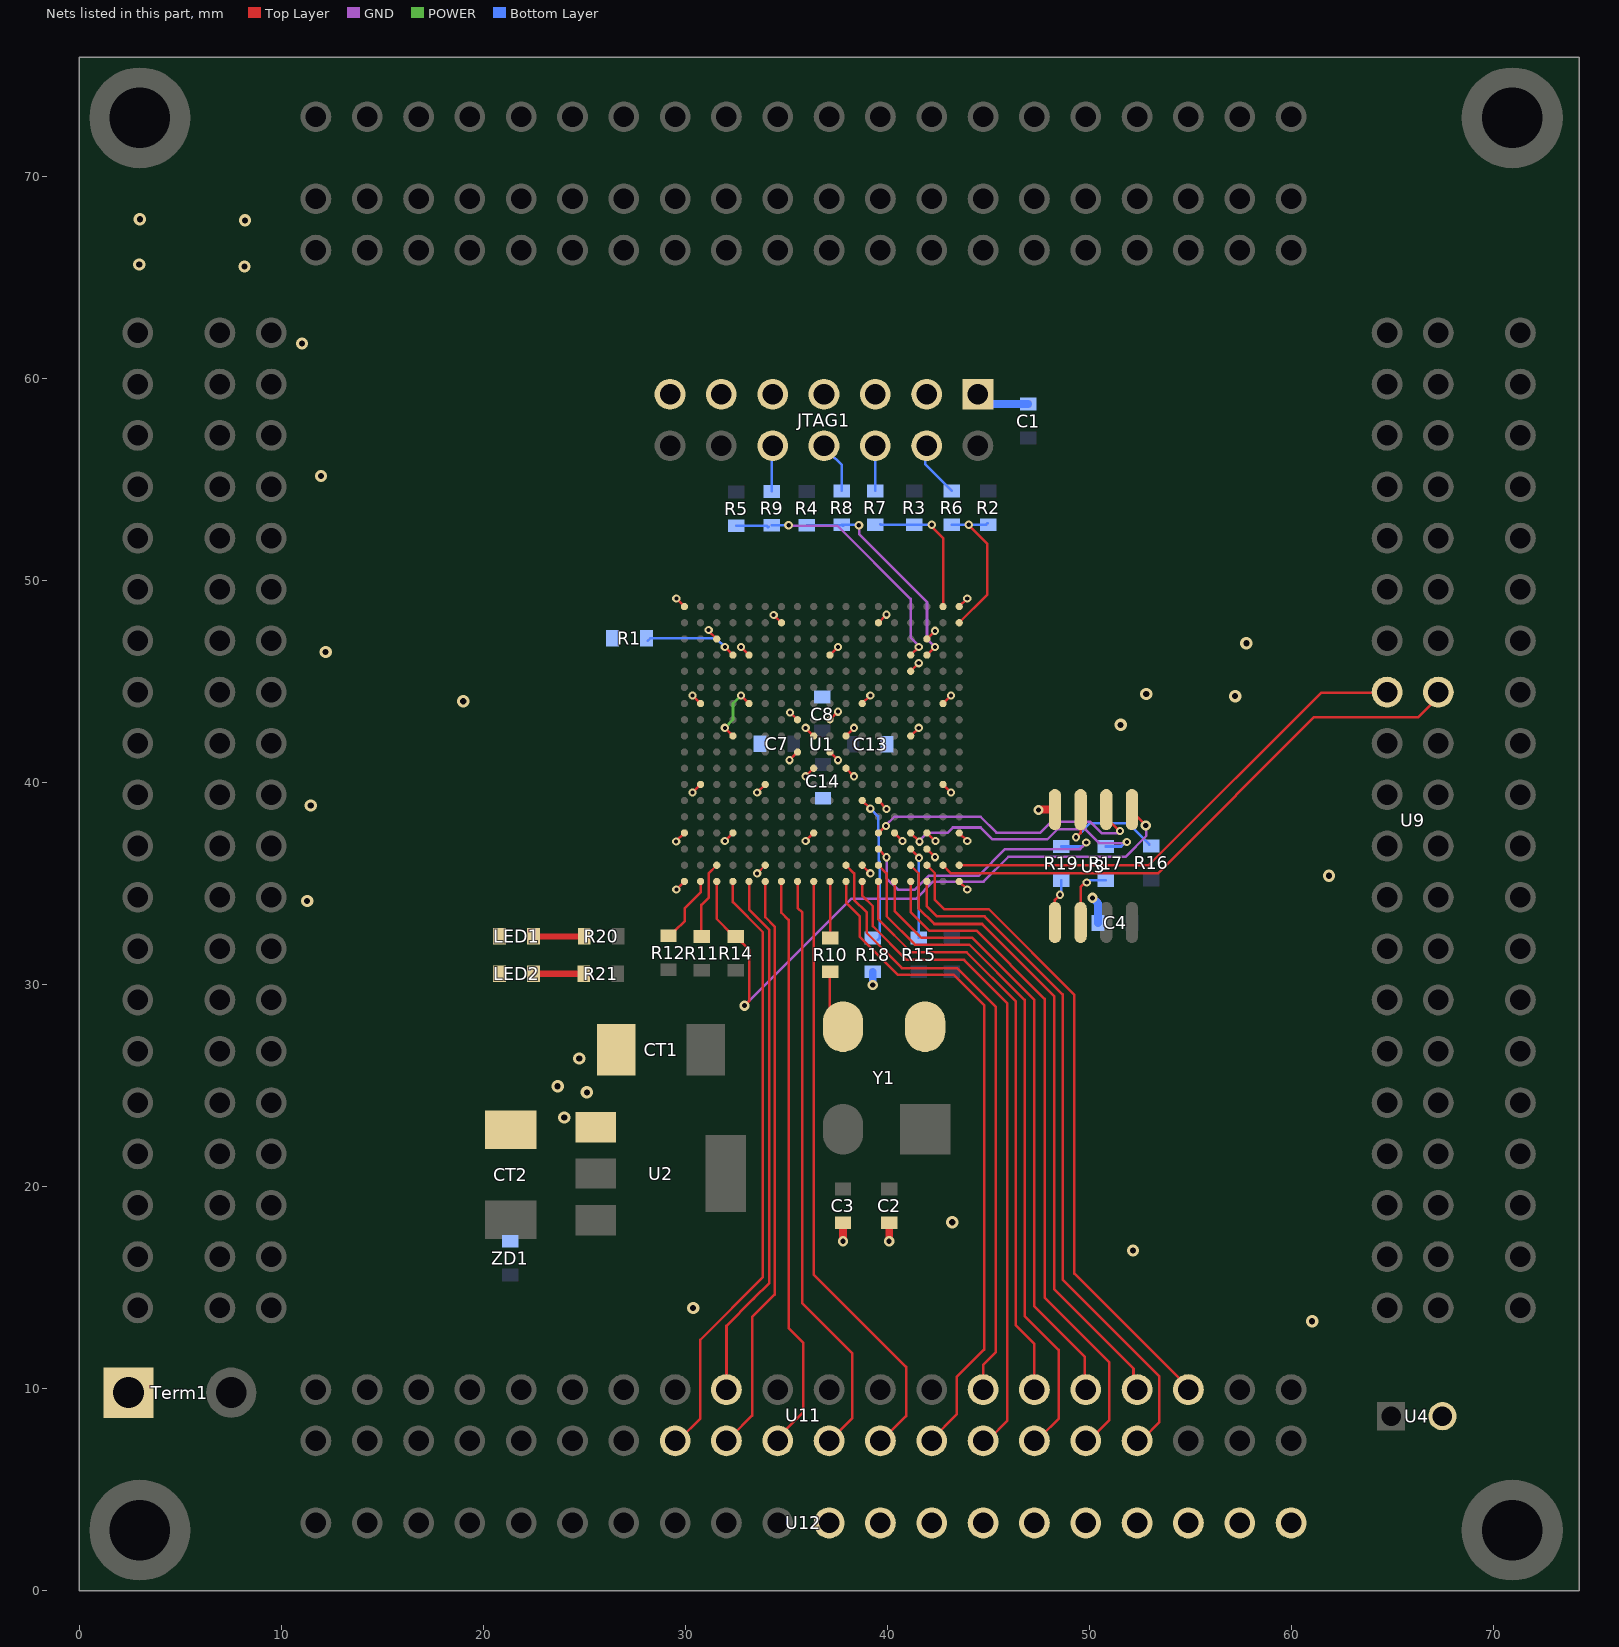
[diagram p0: the nets of this part, all layers, seen from the top]
# Altium PCB MISC103828.PcbDoc (part 4 of 4)
Units mm, origin at the board's own origin, x right, y up, seen from the top; angles counter-clockwise.
Board outline 74.24 x 75.89 mm, 4 copper layers (Top Layer, GND, POWER, Bottom Layer); 49 components, 246 nets, 670 pads, 283 vias.

## Via types
v1: diameter 0.406, hole 0.203, Top Layer to Bottom Layer, 221 vias
v2: diameter 0.61, hole 0.305, Top Layer to Bottom Layer, 43 vias
v3: diameter 0.508, hole 0.254, Top Layer to Bottom Layer, 16 vias
v4: diameter 0.432, hole 0.229, Top Layer to Bottom Layer, 3 vias

## Nets (pads, with @x,y where several pads share a name; then routed paths per layer and width w, separated by ;. In a path a pad name is that pad's centre, name@x,y a point inside that pad or via, vN(x,y) a via of type N, cw(c..) or ccw(c..) an arc to the next point about the centre after c; other vN are vias at no path point) (continued)
F_U11: U1.U11 U11.28 | length 30.9
  Top Layer w0.127: U1.U11@37.947,35.903 38.351,35.499 38.351,34.191 38.964,33.579 38.964,32.563 40.716,30.81 43.434,30.81 45.364,28.88 45.364,11.811 44.729,11.176 U11.28@44.729,9.957
F_U13: U1.U13 U11.29 | length 34
  Top Layer w0.127: U1.U13@39.547,35.903 39.951,35.499 39.951,33.378 41.351,31.979 44.044,31.979 46.787,29.235 46.787,15.037 ; 46.787,14.961 46.787,15.037 ; U11.29@47.6,7.645 48.463,8.509 48.463,11.913 46.787,13.589 46.787,15.037
F_U15: U1.U15 U11.34 | length 31.8
  Top Layer w0.127: U1.U15@41.147,35.903 41.543,35.508 41.543,33.768 42.316,32.995 44.679,32.995 48.26,29.413 48.26,14.91 52.172,10.998 U11.34@52.172,10.033
F_U16: U1.U16 U11.36 | length 32.2
  Top Layer w0.127: U1.U16@41.947,35.903 42.343,35.508 42.343,34.187 42.799,33.731 45.009,33.731 49.251,29.489 49.251,15.697 U11.36@54.686,10.262
F_U17: U1.U17 U9.16 | length 28.3
  Top Layer w0.127: U1.U17@42.747,35.903 43.151,35.499 53.381,35.499 61.112,43.231 66.269,43.231 U9.16@67.285,44.247
F_U18: U1.U18 U9.15 | length 24.7
  Top Layer w0.127: U1.U18@43.547,35.903 52.921,35.903 61.468,44.45 U9.15@64.668,44.45
F_V4: U1.V4 U11.15 | length 29.9
  Top Layer w0.127: U11.15@29.693,7.493 30.734,8.534 30.734,12.421 33.833,15.519 33.833,32.588 32.347,34.074 U1.V4@32.347,35.103
F_V5: U1.V5 U11.18 | length 26.4
  Top Layer w0.127: U11.18@32.029,9.957 32.029,13.106 33.35,14.427 33.401,14.478 34.138,15.215 34.138,32.715 33.147,33.705 U1.V5@33.147,35.103
F_V6: U1.V6 U11.17 | length 28.5
  Top Layer w0.127: U11.17@32.309,7.671 33.299,8.661 33.299,13.538 34.417,14.656 34.417,32.868 33.947,33.337 U1.V6@33.947,35.103
F_V7: U1.V7 U11.19 | length 28.1
  Top Layer w0.127: U1.V7@34.747,35.103 34.747,33.553 35.103,33.198 35.103,13.005 35.839,12.268 35.839,8.839 U11.19@34.849,7.849
F_V8: U1.V8 U11.21 | length 28.9
  Top Layer w0.127: U1.V8@35.547,35.103 35.547,33.795 35.789,33.553 35.789,14.757 ; 35.789,14.63 35.789,14.757 ; U11.21@37.516,7.798 38.252,8.534 38.252,11.76 35.789,14.224 35.789,14.757
F_V9: U1.V9 U11.23 | length 29.7
  Top Layer w0.127: 36.347,16.459 36.347,16.51 ; U1.V9@36.347,35.103 36.347,16.51 ; U11.23@39.98,7.696 40.919,8.636 40.919,11.074 36.347,15.646 36.347,16.51
F_V11: U1.V11 U11.25 | length 33.2
  Top Layer w0.127: U1.V11@37.947,35.103 37.947,34.062 38.633,33.376 38.633,32.36 40.513,30.48 43.282,30.48 44.78,28.981 44.78,11.938 43.434,10.592 43.434,8.738 U11.25@42.164,7.468
F_V12: U1.V12 U11.27 | length 32.6
  Top Layer w0.127: U1.V12@38.747,35.103 38.747,34.405 39.268,33.884 39.268,32.893 40.945,31.217 43.79,31.217 45.923,29.083 45.923,8.407 U11.27@45.034,7.518
F_V13: U1.V13 U11.30 | length 30
  Top Layer w0.127: U1.V13@39.547,35.103 39.547,33.224 41.173,31.598 43.917,31.598 46.355,29.159 46.355,13.716 ; 46.355,13.589 46.355,13.716 ; U11.30@47.269,10.084 47.269,12.217 46.355,13.132 46.355,13.716
F_V14: U1.V14 U11.32 | length 30.3
  Top Layer w0.127: U1.V14@40.347,35.103 40.347,33.643 41.681,32.309 44.196,32.309 47.269,29.235 47.269,14.072 49.759,11.582 U11.32@49.759,10.16
F_V15: U1.V15 U11.31 | length 33.4
  Top Layer w0.127: U1.V15@41.147,35.103 41.147,33.579 42.062,32.664 44.399,32.664 47.777,29.286 47.777,14.503 50.978,11.303 50.978,8.458 U11.31@50.063,7.544
F_V16: U1.V16 U11.33 | length 34
  Top Layer w0.127: U1.V16@41.947,35.103 41.947,33.872 42.443,33.376 44.806,33.376 48.666,29.515 48.666,15.392 53.442,10.617 53.442,8.331 U11.33@52.68,7.569
FPGA_CCLK: R17.1 U1.R15 | length 13
  Top Layer w0.127: U1.R15@41.147,37.503 v1(41.58,37.071)
  GND w0.127: v1(41.58,37.071) 41.547,37.103 41.947,37.503 42.53,37.503 42.596,37.503 42.964,37.503 43.231,37.77 44.602,37.77 45.187,37.186 47.904,37.186 48.4,37.681 49.797,37.681 50.495,36.982 51.765,36.982 v1(51.841,37.059)
  Bottom Layer w0.127: R17.1@50.8,36.83 51.562,36.83 v1@51.765,37.033
FPGA_CSO_B: R14.2 U1.V3 U3.1 | length 31.8
  Top Layer w0.127: U1.V3@31.547,35.103 31.547,33.248 32.309,32.487 R14.2@32.512,32.487 ; R14.2@32.487,32.385 33.147,31.725 33.147,29.185 v3(32.918,28.956) ; U3.1@52.095,38.659 52.095,38.557 v3(52.781,37.871)
  GND w0.127: v3(32.918,28.956) 38.202,34.239 41.402,34.239 42.26,35.097 44.749,35.097 45.974,36.322 51.765,36.322 52.807,37.363 v3@52.807,37.821
FPGA_DIN: U1.R13 U3.2 | length 14.4
  Top Layer w0.127: U1.R13@39.547,37.503 39.561,37.503 v1@39.878,37.821 ; v1(39.929,37.846) v1@39.954,37.821 ; U3.2@50.825,38.659 50.825,38.252 v1@51.46,37.617
  GND w0.127: v1(39.929,37.846) v1@39.954,37.821 ; v1@39.929,37.897 40.335,38.303 44.602,38.303 45.39,37.516 ; 45.39,37.51 47.543,37.51 48.082,38.049 50.038,38.049 50.597,37.49 51.41,37.49 v1(51.511,37.592)
FPGA_INIT_B: R11.2 U1.U3 | length 3.7
  Top Layer w0.127: R11.2@30.836,32.512 30.785,32.563 30.785,33.934 31.143,34.293 31.143,35.499 U1.U3@31.547,35.903
FPGA_M0: R15.2 U1.T15 | length 4.5
  Top Layer w0.127: U1.T15@41.147,36.703 41.554,36.296 v1(41.554,36.271)
  Bottom Layer w0.127: R15.2@41.554,32.309 v1@41.554,36.22
FPGA_M1: R18.2 U1.N12 | length 7.3
  Top Layer w0.127: U1.N12@38.747,39.103 v1(39.147,38.703)
  Bottom Layer w0.127: v1(39.147,38.703) 39.535,38.316 39.535,38.049 39.535,37.338 39.56,37.313 39.56,36.134 39.611,36.083 39.611,32.296 R18.2@39.522,32.207
FPGA_MOSI: R19.1 U1.T13 | length 14
  Top Layer w0.127: U1.T13@39.547,36.703 v1(39.954,36.297)
  GND w0.127: v1(39.954,36.297) 39.954,35.255 40.513,34.696 41.351,34.696 42.037,35.382 44.501,35.382 45.822,36.703 49.53,36.703 v1@49.86,37.033 ; v1@49.797,37.033 v1(49.835,37.033)
  Bottom Layer w0.127: R19.1@48.59,36.83 49.632,36.83 v1@49.784,36.982
GND: C1.1 C2.1 C3.1 C4.2 C7.1 C8.1 C13.1 C14.1 CT1.2 CT2.2 JTAG1.1 JTAG1.3 JTAG1.5 JTAG1.7 JTAG1.9 JTAG1.11 JTAG1.13 LED1.K LED2.K R1.1 R18.1 Term1.1 U1.A1 U1.A18 U1.B7 U1.B13 U1.C3 U1.C16 U1.D5 U1.D10 U1.E15 U1.G2 U1.G5 U1.G12 U1.G17 U1.H8 U1.H10 U1.J4 U1.J9 U1.J11 U1.J15 U1.K8 U1.K10 U1.L9 U1.L11 U1.M2 U1.M6 U1.M17 U1.N13 U1.R1 U1.R4 U1.R9 U1.R14 U1.R16 U1.R18 U1.T16 U1.U6 U1.U12 U1.V1 U1.V18 U2.1 U3.4 U4.2 U12.11 U12.12 U12.13 U12.14 U12.15 U12.16 U12.17 U12.18 U12.19 U12.20 Y1.2 ZD1.1 | length 30.4
  Top Layer w0.127: v1(29.54,37.084) 29.54,37.096 U1.R1@29.947,37.503 ; v1(29.547,34.703) U1.V1@29.947,35.103 ; v1(29.547,49.103) U1.A1@29.947,48.703 ; v1(30.347,39.503) U1.M2@30.747,39.903 ; v1(30.347,44.303) U1.G2@30.747,43.903 ; v1(31.147,47.542) 31.147,47.503 U1.C3@31.547,47.103 ; v1(31.947,37.103) U1.R4@32.347,37.503 ; v1(31.947,42.703) U1.J4@32.347,42.303 ; v1(32.747,44.303) U1.G5@33.147,43.903 ; v1(32.747,46.703) U1.D5@33.147,46.303 ; v1(33.547,35.503) U1.U6@33.947,35.903 ; v1(33.547,39.503) U1.M6@33.947,39.903 ; v1(34.366,48.285) U1.B7@34.747,47.903 ; v1(35.147,41.103) U1.K8@35.547,41.503 ; v1(35.179,43.459) 35.179,43.472 U1.H8@35.547,43.103 ; v1(35.947,37.103) U1.R9@36.347,37.503 ; v1(35.947,40.303) U1.L9@36.347,40.703 ; v1(35.947,42.703) U1.J9@36.347,42.303 ; U1.K10@37.147,41.503 v1(37.547,41.103) ; U1.H10@37.147,43.103 v1(37.547,43.503) ; U1.D10@37.147,46.303 v1(37.547,46.703) ; U1.L11@37.947,40.703 v1(38.347,40.303) ; U1.J11@37.947,42.303 v1(38.347,42.703) ; U1.U12@38.747,35.903 v1(39.147,35.503) ; U1.G12@38.747,43.903 v1(39.147,44.303) ; U1.N13@39.547,39.103 39.954,38.697 v1(39.954,38.684) ; U1.B13@39.547,47.903 v1(39.947,48.303) ; U1.R14@40.347,37.503 v1(40.747,37.103) ; U1.J15@41.147,42.303 v1(41.547,42.703) ; U1.E15@41.147,45.503 v1(41.547,45.903) ; U1.T16@41.947,36.703 v1(42.347,36.303) ; U1.R16@41.947,37.503 42.347,37.103 42.353,37.109 v1(42.367,37.109) ; U1.C16@41.947,47.103 v1(42.347,47.503) ; U1.M17@42.747,39.903 v1(43.147,39.503) ; U1.G17@42.747,43.903 v1(43.147,44.303) ; U1.V18@43.547,35.103 v1(43.947,34.703) ; U1.R18@43.547,37.503 v1(43.947,37.103) ; U1.A18@43.547,48.703 v1(43.947,49.103)
  Top Layer w0.381: v3(37.795,17.297) C3.1@37.795,18.212 ; v3(40.081,17.297) C2.1@40.081,18.212 ; v3(47.473,38.633) 47.498,38.659 U3.4@48.285,38.659
  POWER w0.127: v1(31.947,42.703) 32.354,43.11 32.354,43.91 v1(32.747,44.303)
  Bottom Layer w0.381: v3(39.268,29.972) R18.1@39.268,30.632 ; JTAG1.1@44.856,59.004 45.136,58.725 C1.1@46.965,58.725 ; v3(50.14,34.29) 50.419,34.011 C4.2@50.419,33.045
  other v2: 61.011,13.335 30.378,13.995 52.146,16.84 43.205,18.237 24.003,23.419 25.121,24.663 23.673,24.968 24.74,26.34 11.278,34.138 61.849,35.382 11.455,38.862 51.537,42.85 18.999,44.018 57.201,44.272 52.807,44.374 12.192,46.457 57.76,46.888 11.963,55.169 11.024,61.722 8.179,65.532 2.972,65.634 8.204,67.818 2.997,67.869
NetJTAG1_4: JTAG1.4 R6.2 | length 2.5
  Bottom Layer w0.127: JTAG1.4@41.859,56.388 41.859,55.753 R6.2@43.18,54.432
NetJTAG1_6: JTAG1.6 R7.2 | length 1.8
  Bottom Layer w0.127: JTAG1.6@39.37,56.236 39.395,56.21 R7.2@39.395,54.432
NetJTAG1_8: JTAG1.8 R8.2 | length 2.2
  Bottom Layer w0.127: JTAG1.8@37.109,56.337 37.744,55.702 R8.2@37.744,54.432
NetJTAG1_10: JTAG1.10 R9.2 | length 2
  Bottom Layer w0.127: JTAG1.10@34.214,56.388 34.265,56.337 R9.2@34.265,54.407
NetLED1_A: LED1.A R20.1 | length 2.4
  Top Layer w0.127: LED1.A@22.555,32.36 LED1.A@22.581,32.385
  Top Layer w0.305: LED1.A@22.581,32.385 R20.1@24.994,32.385
NetLED2_A: LED2.A R21.1 | length 2.4
  Top Layer w0.127: LED2.A@22.555,30.607 LED2.A@22.631,30.531
  Top Layer w0.305: LED2.A@22.631,30.531 R21.1@24.968,30.531
NetR1_2: R1.2 U1.D4 | length 4.6
  Top Layer w0.127: v1(31.947,46.703) U1.D4@32.347,46.303
  Bottom Layer w0.127: R1.2@28.143,47.015 28.258,47.13 31.521,47.13 v1(31.947,46.703)
NetR10_1: R10.1 Y1.3 | length 2.5
  Top Layer w0.127: R10.1@37.186,30.582 37.135,30.531 37.135,28.88 Y1.3@37.719,28.296
NetR16_1: R16.1 U3.3 | length 5.9
  Top Layer w0.127: v1(49.327,37.287) 49.327,37.262 49.555,37.49 U3.3@49.555,38.659
  Bottom Layer w0.127: v1@49.352,37.313 v1(49.327,37.287) 50.025,37.986 51.905,37.986 R16.1@52.959,36.932
NetR17_2: R17.2 U3.6 | length 3
  Top Layer w0.127: U3.6@49.555,33.071 49.555,34.823 v1@49.784,35.052
  Bottom Layer w0.127: v1@49.886,35.077 49.962,35.154 R17.2@50.8,35.154
  other v1: 49.86,35.052
NetR19_2: R19.2 U3.5 | length 2.1
  Top Layer w0.127: U3.5@48.285,33.071 48.285,34.188 v1(48.539,34.442)
  Bottom Layer w0.127: v1@48.59,34.519 R19.2@48.59,35.154
PROGRAM_B: R12.2 U1.V2 | length 3
  Top Layer w0.127: R12.2@29.464,32.639 29.972,33.147 29.972,33.782 30.747,34.557 U1.V2@30.747,35.103
SYS_CLK: R10.2 U1.V10 | length 2.8
  Top Layer w0.127: R10.2@37.16,32.309 U1.V10@37.16,35.077
TCK: R3.2 R7.1 U1.A17 | length 6.7
  Top Layer w0.127: v1@42.24,52.603 42.747,52.096 U1.A17@42.747,48.703
  Bottom Layer w0.127: R7.1@39.649,52.781 39.675,52.756 R3.2@41.326,52.756 42.164,52.756 v1@42.215,52.807
  other v1: 42.189,52.756
TDI: R5.2 R9.1 U1.D15 | length 13.1
  Top Layer w0.127: U1.D15@41.147,46.303 v1(41.547,46.703)
  GND w0.127: v4(35.103,52.73) v4@35.154,52.68 ; v4@35.179,52.705 37.516,52.705 41.141,49.08 41.141,48.514 41.141,47.175 v1@41.58,46.736
  Bottom Layer w0.127: R5.2@32.512,52.705 34.011,52.705 34.087,52.629 R9.1@34.112,52.654 ; R9.1@34.265,52.73 v4(35.103,52.73)
TDO: R4.2 R8.1 U1.D16 | length 10.7
  Top Layer w0.127: U1.D16@41.947,46.303 v1(42.347,46.703)
  GND w0.127: v4@38.608,52.654 38.608,52.273 41.954,48.928 41.954,47.097 v1(42.347,46.703)
  Bottom Layer w0.127: R4.2@35.992,52.73 37.77,52.73 R8.1@37.795,52.705 ; R8.1@37.744,52.756 38.557,52.756 v4(38.583,52.73)
TMS: R2.2 R6.1 U1.B18 | length 7.6
  Top Layer w0.127: U1.B18@43.547,47.903 44.933,49.289 44.933,51.816 v4@44.018,52.73
  Bottom Layer w0.127: R6.1@43.18,52.756 v4(44.018,52.756) 44.882,52.756 R2.2@44.958,52.832
pads on no net: JTAG1.12 JTAG1.14 U1.F16 U1.F17 U1.L12 U1.L13 U1.P13 U1.U5 U9.23 U11.35 Y1.1

## Polygon pours and split planes (outlines as drawn)
GND on Top Layer "TopLayer-No Net" (solid, remove dead copper): 0.889,68.428 0.889,7.103 1.321,6.671 1.626,6.367 2.337,6.367 5.715,6.367 6.477,5.605 6.579,5.503 6.579,1.363 7.239,0.702 9.677,0.702 66.65,0.702 66.904,0.956 66.904,1.439 66.904,4.919 68.758,6.773 68.759,6.774 72.289,6.774 73.254,7.738 73.254,14.647 73.254,68.317 72.568,69.003 69.52,69.003 67.361,71.162 67.361,73.981 66.446,74.896 7.899,74.896 7.137,74.134 7.137,71.264 4.902,69.028 1.473,69.028 0.889,68.444 0.889,68.428
+3.3V on Top Layer "TopLayer-No Net" (solid, remove dead copper, pour order 1000): 5.486,10.643 5.486,8.687 5.747,8.433 9.858,8.433 10.092,8.661 10.352,8.915 10.352,9.855 10.352,10.846 10.586,11.074 10.95,11.43 11.939,11.43 15.243,11.43 16.206,12.37 18.47,14.58 21.332,14.58 26.223,14.58 26.405,14.757 26.848,15.189 26.848,16.231 26.848,18.948 26.692,19.101 26.64,19.152 23.361,19.152 23.127,19.152 22.893,19.38 22.815,19.456 22.06,19.456 13.006,19.456 10.742,17.247 10.69,17.196 10.69,16.18 10.118,15.621 9.988,15.494 8.973,15.494 5.929,15.494 5.616,15.189 5.486,15.062 5.486,10.643
+1.2V on Top Layer "TopLayer-No Net" (solid, remove dead copper, pour order 1001): 24.308,21.209 24.308,19.99 24.46,19.837 24.511,19.787 24.536,19.761 27.534,19.761 28.727,18.567 29.235,18.059 31.242,18.059 32.817,18.059 32.944,18.186 33.096,18.339 33.096,18.796 33.096,27.559 32.664,27.991 32.512,28.143 32.334,28.321 30.175,28.321 30.124,28.321 29.87,28.067 29.743,27.94 29.743,27.28 29.743,22.835 29.159,22.25 28.473,21.565 27.076,21.565 24.409,21.565 24.308,21.463 24.308,21.184
+3.3V on POWER "TopLayer-No Net" (solid, remove dead copper): 0.889,68.402 0.889,7.078 1.321,6.646 1.626,6.341 2.337,6.341 5.715,6.341 6.477,5.579 6.579,5.478 6.579,1.337 7.239,0.677 9.677,0.677 66.65,0.677 66.904,0.931 66.904,1.414 66.904,4.893 68.758,6.748 68.759,6.748 72.289,6.748 73.254,7.713 73.254,14.622 73.254,68.292 72.568,68.978 69.52,68.978 67.361,71.137 67.361,73.956 66.446,74.87 7.899,74.87 7.137,74.108 7.137,71.238 4.902,69.003 1.473,69.003 0.889,68.419 0.889,68.402
+1.2V on POWER "TopLayer-No Net" (solid, remove dead copper, pour order 1003): 33.985,44.399 33.985,42.774 33.985,42.748 33.757,42.52 33.68,42.443 31.75,42.443 26.645,42.443 24.943,42.443 24.105,41.605 24.105,25.705 25.451,24.359 26.391,23.419 30.302,23.419 32.537,23.419 33.096,23.978 33.325,24.206 33.325,24.917 33.325,27.356 32.868,27.813 32.106,28.575 31.801,28.575 29.312,28.575 28.651,29.235 27.661,30.226 27.661,38.125 27.661,40.208 28.321,40.869 28.88,41.427 31.648,41.427 34.468,41.427 34.62,41.427 34.722,41.326 34.823,41.224 34.823,40.818 34.823,40.335 34.493,40.005 34.112,39.624 34.112,39.548 34.112,39.319 34.239,39.192 34.392,39.04 34.849,39.04 35.408,39.04 35.585,39.218 35.585,39.421 35.585,39.751 35.712,39.878 36.906,39.878 37.541,39.878 37.821,40.157 37.922,40.259 38.227,40.259 38.684,40.259 38.837,40.107 38.887,40.056 38.887,39.751 38.887,39.395 38.938,39.345 39.04,39.243 39.294,39.243 39.573,39.243 39.726,39.395 39.827,39.497 39.954,39.624 39.954,41.173 39.954,42.037 39.776,42.215 39.675,42.316 39.294,42.316 38.989,42.316 38.862,42.443 38.76,42.545 38.76,42.875 38.76,43.866 38.684,43.942 38.633,43.993 38.202,43.993 37.287,43.993 37.084,44.196 36.576,44.704 36.119,44.704 34.163,44.704 33.985,44.526 33.985,44.399
GND on Bottom Layer "TopLayer-No Net" (solid, remove dead copper): 0.94,68.436 0.94,7.112 1.372,6.68 1.676,6.375 2.388,6.375 5.766,6.375 6.528,5.613 6.629,5.512 6.629,1.372 7.29,0.711 9.728,0.711 66.7,0.711 66.954,0.965 66.954,1.448 66.954,4.928 68.809,6.782 68.81,6.783 72.34,6.783 73.304,7.747 73.304,14.656 73.304,68.326 72.619,69.012 69.571,69.012 67.412,71.171 67.412,73.99 66.497,74.905 7.95,74.905 7.188,74.143 7.188,71.272 4.953,69.037 1.524,69.037 0.94,68.453 0.94,68.436
GND on GND "TopLayer-No Net" (solid, remove dead copper): 0.94,68.428 0.94,7.103 1.372,6.671 1.676,6.367 2.388,6.367 5.766,6.367 6.528,5.605 6.629,5.503 6.629,1.363 7.29,0.702 9.728,0.702 66.7,0.702 66.954,0.956 66.954,1.439 66.954,4.919 68.809,6.773 68.81,6.774 72.34,6.774 73.304,7.738 73.304,14.647 73.304,68.317 72.619,69.003 69.571,69.003 67.412,71.162 67.412,73.981 66.497,74.896 7.95,74.896 7.188,74.134 7.188,71.264 4.953,69.028 1.524,69.028 0.94,68.444 0.94,68.428

## Other copper
Top Layer:
  pour cut-out: 29.21,34.62 29.362,34.468 44.12,34.468 44.323,34.671 44.323,49.124 44.12,49.327 29.362,49.327 29.21,49.174

## Silkscreen, mask and mechanical layers (free items; w line width, h text height)
Mechanical 1:
  circle w0.254: c10.7,-82.087 r1.35
  lines w0.127: 74.244,75.889 0,75.889 0,0 74.244,0 74.244,75.895